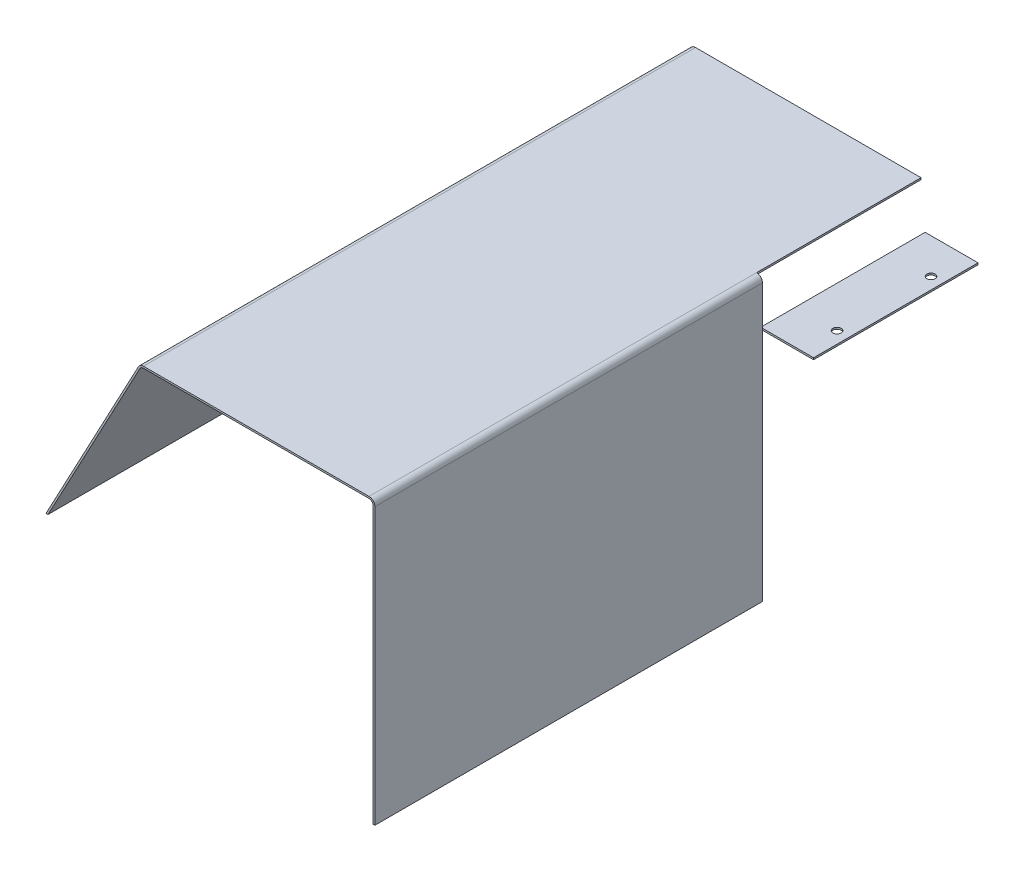
from build123d import *

# Parameters (mm, degrees)
BOSS_EXTRUDE1_DEPTH = 470
SKETCH2_W           = 259.384711363
SKETCH2_H           = 314.468537248
CUT_EXTRUDE3_DEPTH  = 1.5
SKETCH5_W           = 57.928223487
SKETCH5_H           = 140
CUT_EXTRUDE9_DEPTH  = 58.5
SKETCH7_W           = 48.5
SKETCH7_H           = 140
BOSS_EXTRUDE3_DEPTH = 1.5
MOVE_FACE1_BY       = 3.5
SKETCH9_R           = 3.5
CUT_EXTRUDE10_DEPTH = 1.5


with BuildPart() as part:
    # Sketch1 → Boss-Extrude1 (new body)
    with BuildSketch(Plane.XY):
        with BuildLine():
            Line((0, 0), (78.588235294, 147.352941176))
            ThreePointArc((78.588235294, 147.352941176), (80.427521223, 149.287464629), (83, 150))
            Line((83, 150), (275, 150))
            ThreePointArc((275, 150), (278.535533906, 148.535533906), (280, 145))
            Line((280, 145), (280, -90))
            Line((280, -90), (278.5, -90))
            Line((278.5, -90), (278.5, 145))
            ThreePointArc((278.5, 145), (277.474873734, 147.474873734), (275, 148.5))
            Line((275, 148.5), (83, 148.5))
            ThreePointArc((83, 148.5), (81.199264856, 148.00122524), (79.911764706, 146.647058824))
            Line((79.911764706, 146.647058824), (1.7, 0))
            Line((1.7, 0), (0, 0))
        make_face()
    extrude(amount=BOSS_EXTRUDE1_DEPTH)

    # Sketch2 → Cut-Extrude3 (cut)
    with BuildSketch(Plane.ZY.offset(-278.5)):
        with Locations((10.307644318, -12.234268624)):
            Rectangle(SKETCH2_W, SKETCH2_H)
    extrude(amount=-CUT_EXTRUDE3_DEPTH, mode=Mode.SUBTRACT)

    # Sketch5 → Cut-Extrude9 (cut)
    with BuildSketch(Plane(origin=(0, 150, 0), x_dir=(1, 0, 0), z_dir=(0, 1, 0))):
        with Locations((303.964111743, -70)):
            Rectangle(SKETCH5_W, SKETCH5_H)
    extrude(amount=-CUT_EXTRUDE9_DEPTH, mode=Mode.SUBTRACT)

    # Sketch7 → Boss-Extrude3 (add)
    with BuildSketch(Plane(origin=(0, 110, 0), x_dir=(1, 0, 0), z_dir=(0, 1, 0))):
        with Locations((299.25, -70)):
            Rectangle(SKETCH7_W, SKETCH7_H)
    extrude(amount=BOSS_EXTRUDE3_DEPTH)

    # Move Face1: a face moved inward by 3.5
    extrude(part.faces().sort_by_distance((275, 110.75, 70))[0], amount=MOVE_FACE1_BY, dir=(1, 0, 0), mode=Mode.SUBTRACT)

    # Sketch9 → Cut-Extrude10 (cut)
    with BuildSketch(Plane(origin=(0, 111.5, 0), x_dir=(1, 0, 0), z_dir=(0, 1, 0))):
        with Locations(Location((313.5, -30, 0), (0, 0, 270))):
            Circle(SKETCH9_R)
        with Locations(Location((313.5, -110, 0), (0, 0, 270))):
            Circle(SKETCH9_R)
    extrude(amount=-CUT_EXTRUDE10_DEPTH, mode=Mode.SUBTRACT)


solid = part.part
